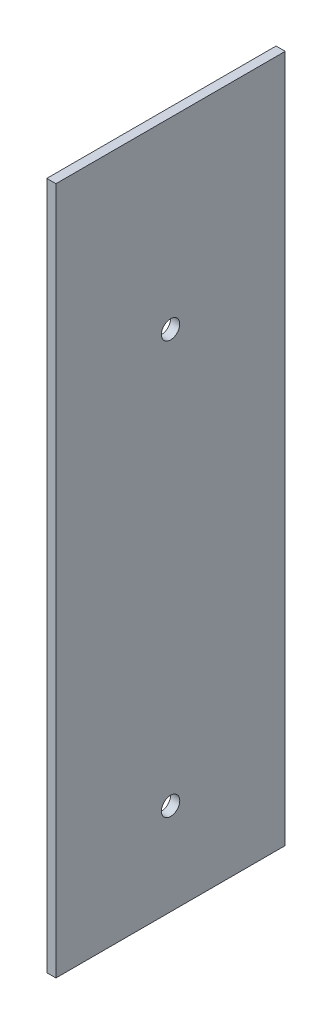
from build123d import *

# Parameters (mm, degrees)
SKETCH_1_W          = 2
SKETCH_1_H          = 180
EXTRUDE_1_DEPTH     = 50
SKETCH_2_R          = 2
CUT_EXTRUDE_1_DEPTH = 20
SKETCH_3_R          = 2
CUT_EXTRUDE_2_DEPTH = 10
SKETCH_4_W          = 190.004489292
SKETCH_4_H          = 85.174426234
CUT_EXTRUDE_3_DEPTH = 10


with BuildPart() as part:
    # 草图1 → 凸台-拉伸1 (new body)
    with BuildSketch(Plane.XY):
        Rectangle(SKETCH_1_W, SKETCH_1_H)
    extrude(amount=EXTRUDE_1_DEPTH)

    # 草图2 → 切除-拉伸1 (cut)
    with BuildSketch(Plane(origin=(1, 0, 0), x_dir=(0, 0, -1), z_dir=(1, 0, 0))):
        with Locations((-25, -40)):
            Circle(SKETCH_2_R)
    extrude(amount=-CUT_EXTRUDE_1_DEPTH, mode=Mode.SUBTRACT)

    # 草图3 → 切除-拉伸2 (cut)
    with BuildSketch(Plane(origin=(1, 0, 0), x_dir=(0, 0, -1), z_dir=(1, 0, 0))):
        with Locations((-25, 50)):
            Circle(SKETCH_3_R)
    extrude(amount=-CUT_EXTRUDE_2_DEPTH, mode=Mode.SUBTRACT)

    # 草图4 → 切除-拉伸3 (cut)
    with BuildSketch(Plane.ZY.offset(1)):
        with Locations((56.530917404, -102.587213117)):
            Rectangle(SKETCH_4_W, SKETCH_4_H)
    extrude(amount=-CUT_EXTRUDE_3_DEPTH, mode=Mode.SUBTRACT)


solid = part.part
